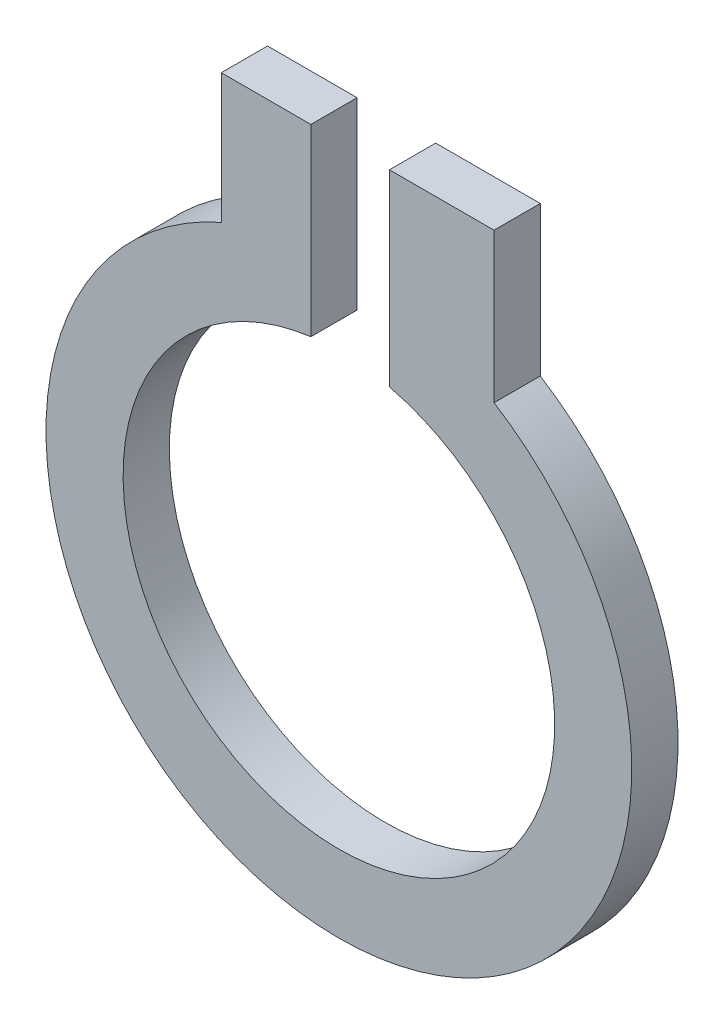
from build123d import *

# Parameters (mm, degrees)
BOSS_EXTRUDE1_DEPTH = 0.6


with BuildPart() as part:
    # Sketch1 → Boss-Extrude1 (new body)
    with BuildSketch(Plane.XY):
        with BuildLine():
            Line((0.655924801, 2.722087922), (0.655924801, 5.162028968))
            Line((0.655924801, 5.162028968), (2.012866642, 5.162028968))
            Line((2.012866642, 5.162028968), (2.012866642, 3.223099112))
            ThreePointArc((2.012866642, 3.223099112), (-0.275338884, -3.790011675), (-1.525882777, 3.480184155))
            Line((-1.525882777, 3.480184155), (-1.525882777, 5.162028968))
            Line((-1.525882777, 5.162028968), (-0.363562636, 5.162028968))
            Line((-0.363562636, 5.162028968), (-0.363562636, 2.776296492))
            ThreePointArc((-0.363562636, 2.776296492), (-0.148672631, -2.796050151), (0.655924801, 2.722087922))
        make_face()
    extrude(amount=BOSS_EXTRUDE1_DEPTH)


solid = part.part
